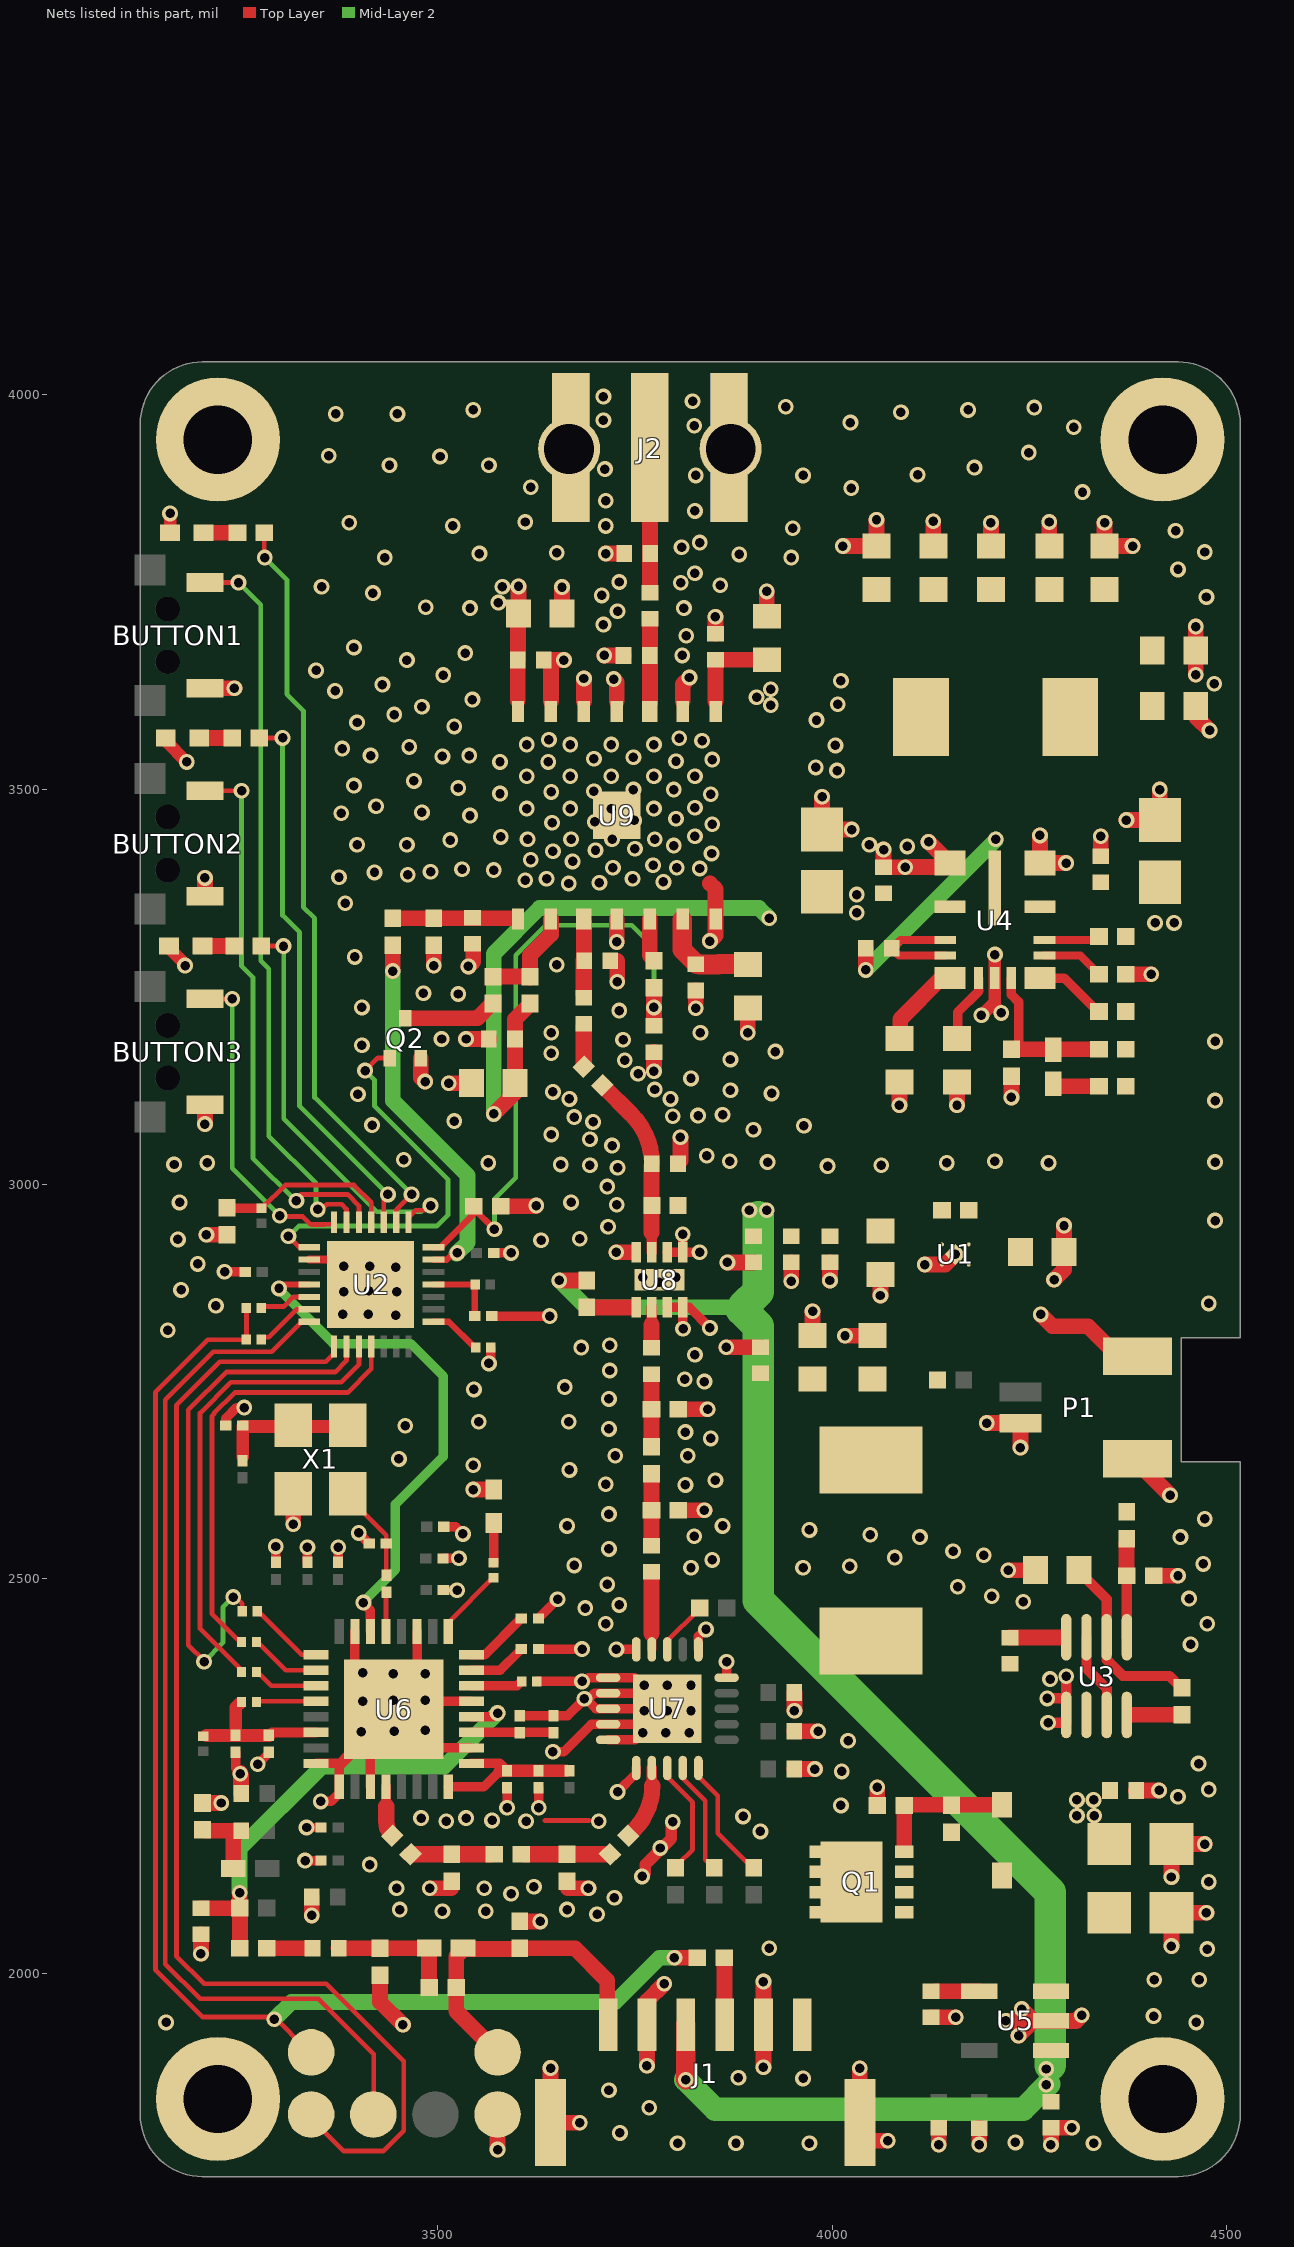
[diagram p0: the nets of this part, all layers, seen from the top]
# Altium PCB MISC62792.PcbDoc (part 2 of 2)
Units mil, origin at the board's own origin, x right, y up, seen from the top; angles counter-clockwise.
Board outline 1393.7 x 2299.21 mil, 4 copper layers (Top Layer, Mid-Layer 1, Mid-Layer 2, Bottom Layer); 176 components, 94 nets, 498 pads, 570 vias.

## Via types
v1: diameter 20, hole 12, Top Layer to Bottom Layer, tented both sides, 570 vias

## Nets (pads, with @x,y where several pads share a name; then routed paths per layer and width w, separated by ;. In a path a pad name is that pad's centre, name@x,y a point inside that pad or via, vN(x,y) a via of type N, cw(c..) or ccw(c..) an arc to the next point about the centre after c; other vN are vias at no path point) (continued)
GND: BUTTON1.1 BUTTON2.1 BUTTON3.1 C1.2 C2.2 C3.2 C4.2 C5.1 C7.1 C8.2 C9.2 C10.2 C11.2 C12.2 C13.2 C14.2 C15.2 C16.2 C17.2 C18.2 C19.2 C20.2 C21.2 C22.2 C23.2 C24.2 C25.2 C26.2 C27.2 C28.1 C29.2 C30.2 C31.1 C32.1 C33.1 C34.1 C35.2 C36.2 C37.1 C38.2 C39.1 C47.2 C50.2 C51.1 C52.2 C53.1 C54.2 C55.2 C56.1 C57.1 C58.1 C59.1 C60.1 C61.1 C62.1 C63.1 C64.2 C65.2 C67.2 C68.1 C70.1 C71.1 C72.1 C73.2 C74.2 C75.2 C76.2 C78.2 C80.1 C81.2 C82.2 C83.2 C84.2 J1.2 J1.5 J1.7 J1.8 J2.2 LED1.2 LED2.2 LED3.2 LED4.2 P1.1 P1.3 P1.4 P2.1 Q2.2 R3.1 R6.1 R12.2 R14.2 R15.2 R21.2 R25.1 R29.2 R31.2 R32.2 R33.2 R45.2 R51.2 R52.2 R53.2 SCREW1.1 SCREW2.1 SCREW3.1 SCREW4.1 SR1.2 U1.2 U1.5 U2.16 U2.29 U3.5 U4.3 U4.9 U4.11 U5.2 U6.8 U6.9 U6.11 U6.18 U6.21 U6.27 U6.31 U6.33 U7.1 U7.10 U7.11 U7.15 U7.16 U7.17 U7.18 U7.19 U7.20 U7.21 U8.3 U8.4 U8.5 U8.6 U8.8 U8.9 U9.4 U9.7 U9.9 U9.11 U9.12 U9.13 U9.15 X1.2 | length 6024.2
  Top Layer w6: 3636,2194 3692,2194
  Top Layer w10: U2.16@3337.26,2904.5 U2.29@3363.5,2904.5
  Top Layer w12: v1(3230,2889) C14.2@3256.4,2889 ; C51.1@3231.55,2694.31 3231.55,2703.31 3245.24,2717 v1(3255,2717) ; C68.1@3244,2280.2 3244,2260 v1@3250,2254 ; v1(3272,2265) 3286,2279 C67.2@3286,2280.2 ; C58.1@3295,2520.8 v1(3295,2541) ; v1(3332,2143) C53.1@3352.2,2143 ; v1(3334,2185) C52.2@3352.2,2185 ; C63.1@3335,2520.8 v1(3335,2540) ; U6.8@3346,2266.1 3376.1,2266.1 U6.33@3386,2276 ; v1(3352,2218) 3365,2218 3375.52,2228.52 U6.9@3375.52,2236.58 3375.52,2262.52 3393,2280 U6.33@3398,2280 ; C64.2@3374,2520.8 v1(3374,2540) ; U6.33@3395.21,2390.21 U6.31@3395.21,2433.42 ; v1(3400,2558.2) C47.2@3413.2,2545 ; U6.11@3414.89,2236.58 U6.33@3414.89,2274.89 ; U6.33@3473.95,2391.95 U6.27@3473.95,2433.42 ; U6.33@3503.16,2344.84 U6.21@3542.84,2344.84 ; U6.33@3504.21,2285.79 U6.18@3542.84,2285.79 ; C37.1@3506.8,2526 v1(3527,2526) ; C38.2@3507.26,2485.62 v1(3524.62,2485.62) ; C39.1@3507.8,2566 3523,2566 v1(3532,2557) ; v1(3565,2773) 3567.51,2775.51 R6.1@3567.51,2793 ; C7.1@3568.8,2833 v1(3642,2833) ; C16.2@3570.8,2913 v1(3593,2913) ; v1(3588,2210) C36.2@3588,2235.2 ; C30.2@3604,2326.8 C28.1@3647,2326.8 3664.8,2326.8 v1(3686,2348) ; R25.1@3625.51,2370 v1(3683,2370) ; C29.2@3627.8,2411 v1(3683,2411) ; C32.1@3627.8,2450 v1(3652,2474.2) ; v1(3628,2210) C34.1@3628,2235.2 ; v1(3646,2281) 3660,2281 3694.78,2315.78 U7.19@3715.9,2315.78 U7.21@3749.78,2315.78 ; v1@3687,2371 3690.83,2374.83 U7.16@3715.9,2374.83 3749.83,2374.83 U7.21@3750,2375 ; v1@3691,2345 3700.54,2335.46 U7.18@3715.9,2335.46 U7.21@3750.54,2335.46 ; v1@3693,2350 3698.15,2355.15 U7.17@3715.9,2355.15 U7.21@3750.15,2355.15 ; U7.20@3715.9,2296.09 U7.21@3750.09,2296.09 ; v1(3726.44,2410.56) U7.15@3749,2410.56 ; v1(3728,2230) 3751.63,2253.63 U7.1@3751.63,2260.36 ; U8.3@3790.84,2844.16 3818.84,2844.16 v1(3845,2818) ; U8.6@3790.84,2913.84 v1(3831.84,2913.84) ; U8.4@3810.53,2844.16 3810.53,2817.47 v1(3811,2817) ; U8.5@3810.53,2913.84 v1(3810.53,2936.53) ; U7.11@3830.37,2410.56 3830.37,2427.37 3840,2437 v1(3840,2436) ; U7.10@3866.1,2376 v1(3866.1,2394.9)
  Top Layer w13: v1(4272.41,2348.59) 4296.41,2348.59 U3.5@4296.41,2327.58 ; v1(4273.41,2317.59) 4296.41,2317.59 U3.5@4296.41,2327.58 ; v1(4296.41,2376.59) U3.5@4296.41,2327.58
  Top Layer w15: v1(3759,2123) 3763,2127 3763,2138 3796,2171 v1@3796,2189
  Top Layer w16: LED1.2@3155.61,3565.47 3155.61,3561.39 v1(3182,3535) ; LED3.2@3159.55,3301.69 3159.55,3299.45 3181,3278 v1(3180,3277) ; LED2.2@3161.05,3825.31 v1(3161.05,3849.95) ; v1(4189,3214) 4206.01,3231.01 U4.3@4206.01,3261.16 ; v1(4206.01,3290.99) U4.3@4206.01,3261.16 ; v1(4214,3217) 4206.01,3224.99 U4.3@4206.01,3261.16
  Top Layer w20: v1(3200,2025) C80.1@3200,2049.46 ; R53.2@3202,2216.04 v1(3225.96,2216.04) ; v1(3205.14,3076.14) BUTTON3.1@3205.14,3100.9 ; BUTTON2.1@3205.14,3364.68 v1(3205.14,3388.14) ; BUTTON1.1@3205.14,3628.46 v1(3242.54,3628.46) ; v1(3207.04,2935.96) SR1.2@3233,2935.96 ; v1(3250,2253) v1@3250,2254 ; C78.2@3250.88,2228 v1@3250.88,2250.88 ; v1(3317.1,2569.1) X1.2@3317.1,2608 ; v1(3340.46,2073.54) C59.1@3340.46,2097 ; R51.2@3427,1997.96 3427,1964 v1(3456,1935) ; Q2.2@3478.69,3159.61 3478.69,3135.31 v1(3484,3130) ; v1(3490.04,2107.96) R31.2@3517,2107.96 ; v1(3495,3277) R45.2@3495,3302.96 ; v1(3514,3128) C56.1@3542.9,3128 ; v1(3536,3184) C57.1@3564.92,3184 ; v1(3539,3276) 3545,3282 C5.1@3545,3303.46 ; v1(3545.19,2613.19) LED4.2@3571,2613.19 ; v1(3575.94,1776.94) P2.1@3575.94,1821.38 ; R21.2@3580.04,2972 3624,2972 v1(3625,2973) ; R52.2@3604,2066.04 v1(3629.96,2066.04) ; C54.2@3634.54,3664 v1(3660,3664) ; v1(3643.12,1880.12) J1.8@3643.12,1810.98 v1(3679.98,1810.98) ; U9.13@3643.54,3611.8 C54.2@3643.54,3658.46 ; C55.2@3657.56,3723 v1(3657.56,3756.56) ; R32.2@3665,2107.96 v1(3691.04,2107.96) ; U9.12@3685.27,3611.8 v1(3685.27,3640.73) ; v1(3711,3670) C71.1@3735.46,3670 ; v1(3713,3799) C72.1@3736.46,3799 ; v1(3723,3640) 3727,3636 U9.11@3727,3611.8 ; v1(3726.16,2913.84) U8.8@3746,2913.84 ; v1(3727,3307) U9.4@3727,3336.2 ; v1(3727.54,3256.54) C65.2@3727.54,3283 ; v1(3765.16,1883.16) J1.2@3765.16,1935 3765.16,1965.16 v1(3787,1987) ; v1(3774,3143) C70.1@3774,3167.46 ; C50.2@3807.54,3030 v1(3807.54,3059.54) ; U9.9@3810.46,3611.8 3810.46,3633.46 v1(3819,3642) ; R29.2@3813.04,2587 v1(3838,2587) ; R33.2@3814.04,2715 v1(3842,2715) ; v1(3827,3223) C74.2@3827,3245.46 ; v1(3845,3308) 3852.2,3315.2 U9.7@3852.2,3336.2 3852.2,3373.8 3845,3381 ; C76.2@3852,3697.54 v1(3852,3719) ; v1(3865.54,2793.54) C13.2@3909,2793.54 ; v1(3867.08,2900.92) C33.1@3900,2900.92 ; v1(3893,3192) C73.2@3893,3223.44 ; v1(3912.81,1881.19) J1.5@3912.81,1935 v1(3912.81,1989.81) ; C75.2@3917,3719.56 v1(3917,3751) ; v1(3948,2877) C31.1@3948,2900.92 ; C61.1@3952,2259 v1(3978,2259) ; C60.1@3952,2307 v1(3982,2307) ; v1(3952,2333) C62.1@3952,2356 ; C12.2@3975,2808.56 v1(3975,2839) ; v1(3987,3491) C15.2@3987,3449.37 v1(4024.63,3449.37) ; v1(3997,2878) C35.2@3997,2900.92 ; v1(4013.44,3808.56) C81.2@4056,3808.56 v1(4056,3842) ; v1(4016.12,2808.12) C11.2@4051,2808.12 ; v1(4034.85,1879.85) J1.7@4034.85,1810.98 4034.85,1788.15 v1(4070.15,1788.15) ; R3.1@4056.96,2213 v1(4056.96,2235.96) ; v1(4061,2859) C3.2@4061,2885.44 ; v1(4065,3424) C17.2@4065,3401.54 v1(4092.54,3401.54) ; v1(4085,3100) C2.2@4085,3129.44 ; v1@4094,3402 4144.08,3402 U4.11@4148.91,3406.84 v1(4122,3433.75) ; v1(4117.2,2898.2) U1.2@4139.07,2898.2 4143.2,2898.2 U1.5@4154,2909 ; C26.2@4125,1944.46 v1(4156.54,1944.46) ; C22.2@4128,3808.56 v1(4128,3840) ; v1(4135,1783) C25.2@4135,1804.46 ; v1(4158,3100) C84.2@4158,3129.44 ; v1(4186.33,1783.33) C24.2@4186.33,1804.18 ; v1(4195.64,2697.36) P1.1@4238.35,2697.36 v1(4238.35,2666.35) ; C82.2@4201,3808.56 v1(4201,3838) ; v1(4220,1940) U5.2@4276.93,1940 ; v1(4223,2511) C1.2@4257.44,2511 ; v1(4227,3110) R14.2@4227,3136.96 ; v1(4236,1921) U5.2@4255,1940 ; v1(4240,1955) U5.2@4255,1940 ; v1(4263.09,3441.91) U4.9@4263.09,3406.84 v1(4296.16,3406.84) ; v1(4264,2835) 4279,2820 4324,2820 4361.99,2782.01 P1.3@4386.97,2782.01 ; C20.2@4275,3808.56 v1(4275,3839) ; v1(4277,1783) C23.2@4277,1804.46 v1(4303.54,1804.46) ; v1(4281,2879) 4293.56,2891.56 C4.2@4293.56,2914 v1(4293.56,2947.56) ; v1(4316,1947) 4309,1940 U5.2@4276.93,1940 ; C18.2@4340,3415.54 v1(4340,3441) ; v1(4345,3838) C27.2@4345,3808.56 v1(4380.44,3808.56) ; R12.2@4372.04,3266 v1(4404,3266) ; v1(4372.63,3461.37) C19.2@4415,3461.37 v1(4415,3500) ; C8.2@4384.91,2232 v1(4414,2232) ; P1.4@4393.06,2646 P1.4@4386.97,2652.09 4386.97,2647.03 v1(4428,2606) ; R15.2@4407.04,2504 v1(4438,2504) ; v1(4429.74,2034.74) C10.2@4429.74,2077 v1(4474,2077) ; v1(4429.74,2122.26) C9.2@4429.74,2164 v1(4472,2164) ; C21.2@4460.56,3606 4460.56,3592.44 v1(4478,3575) ; v1(4460.56,3645.56) C83.2@4460.56,3676 v1(4460.56,3706.56) ; U5.2@4255,1940 U5.2@4276.93,1940
  other v1: 3804,1785 3878,1785 3971,1785 4331,1785 4232,1786 3731,1798 3768,1830 3717,1852 3963,1867 3881,1868 3156,1938 4461,1938 4407,1946 4408,1992 4465,1992 4475,2031 3920,2032 3702,2075 3506,2079 3561,2079 3452,2081 3664,2081 3724,2096 3593,2101 3448,2108 3559,2108 3622,2110 4477,2116 3414,2138 3782,2159 3909,2180 3798,2192 3511,2193 3612,2193 3704,2193 3569,2194 3479,2197 3536,2197 3887,2199 4011,2213 4438,2224 4477,2233 4012,2256 4464,2266 4020,2295 3760,2305 3789,2305 3819,2305 3403,2306 3445,2307 3484,2308 3762,2333 3791,2333 3821,2333 3405,2345 3444,2346 3484,2346 3762,2365 3791,2365 3821,2365 4276,2373 3444,2380 3484,2380 3405,2381 4454,2417 3713,2443 4475,2443 3687,2463 3730,2467 4242,2471 4452,2475 4202,2478 4159,2490 3715,2493 3821,2514 3963,2514 4022,2516 3673,2517 4470,2519 3848,2524 4079,2527 4192,2530 4153,2535 3717,2538 4111,2553 4441,2553 3825,2554 4048,2556 3971,2562 3664,2567 3861,2567 4472,2576 3717,2582 3814,2619 3713,2620 3852,2625 3667,2638 3545,2644 3451,2652 3725,2656 3817,2656 3846,2678 3814,2686 3717,2690 3459,2694 3552,2699 3666,2699 3717,2728 3546,2740 3661,2743 3838,2750 3813,2753 3718,2764 3826,2784 3682,2793 3718,2796 3158,2815 3447,2834 3380,2835 3412,2835 3219,2846 4477,2849 3381,2864 3448,2864 3413,2865 3175,2866 3781,2876 3760,2882 3802,2882 3447,2895 3381,2896 3414,2896 3196,2899 4156,2911 3631,2929 3171,2930 3680,2931 3716,2946 4485,2954 3727,2974 3173,2977 3669,2977 3715,2997 3728,3021 3994,3023 3693,3024 4062,3024 3166,3025 3656,3025 3208,3027 3564,3027 4145,3027 4274,3027 3918,3028 4485,3028 3870,3029 4206,3029 3457,3031 3841,3036 3721,3049 3693,3057 3644,3063 3900,3069 3964,3074 3417,3075 3697,3079 3521,3080 3673,3085 3798,3086 3830,3087 3861,3088 4485,3106 3667,3108 3795,3108 3399,3114 3923,3115 3646,3117 3871,3119 3775,3120 3821,3134 3754,3140 3737,3157 3871,3158 3644,3166 3928,3168 3404,3176 4485,3181 3735,3183 3505,3184 3644,3192 3833,3192 3730,3220 3404,3224 3526,3241 3482,3242 3651,3278 3395,3288 3383,3356 3666,3381 3705,3382 3786,3383 3611,3385 3638,3387 3747,3387 3375,3389 3462,3392 3420,3395 3491,3396 3571,3398 3531,3399 3832,3400 3722,3401 3803,3401 3773,3404 3671,3409 3618,3411 3847,3419 3646,3422 3700,3423 3750,3425 4095,3428 3799,3429 3398,3430 3461,3430 4047,3430 3516,3436 3614,3437 3669,3437 3721,3437 3775,3437 3580,3440 3826,3441 3848,3456 3645,3458 3699,3459 3749,3461 3802,3463 3541,3467 3378,3470 3480,3471 3613,3476 3668,3476 3720,3476 3774,3476 3826,3477 3422,3479 3846,3494 3579,3495 3644,3497 3698,3498 3748,3500 3799,3500 3526,3502 3394,3505 3470,3511 3613,3517 3668,3517 3720,3517 3774,3517 3826,3517 4006,3524 3979,3528 3579,3535 3640,3535 3802,3536 3848,3538 3698,3539 3748,3541 3506,3542 3415,3543 3540,3543 3379,3552 3464,3554 4004,3556 3613,3557 3668,3557 3720,3557 3774,3557 3835,3562 3641,3563 3806,3565 3521,3580 3398,3585 3980,3588 3445,3595 3480,3605 4007,3608 3544,3614 3370,3625 3430,3633 4484,3634 4011,3638 3507,3645 3346,3651 3461,3664 3810,3670 3535,3673 3394,3680 3815,3695 3710,3709 3728,3726 3541,3730 3812,3730 3485,3731 4474,3744 3708,3746 3418,3749 3353,3757 3858,3759 3808,3762 3730,3763 3826,3774 4438,3779 3433,3794 3948,3794 3882,3798 3553,3799 3651,3800 4472,3801 3809,3807 3832,3813 4435,3828 3950,3831 3519,3834 3713,3834 3388,3838 3611,3839 3826,3853 3713,3866 4317,3877 4024,3882 3618,3883 3827,3898 3963,3898 4108,3899 3712,3906 4180,3908 3439,3911 3565,3911 3503,3922 3362,3923 4249,3927 4306,3959 3825,3961 4023,3965 3710,3968 3371,3976 3449,3976 4087,3978 3545,3981 4172,3981 4256,3984 3941,3985 3823,3992 3710,3998
I_RC: P6.1 R4.2 R7.2 R8.2 | length 1715.7
  Top Layer w6: R7.2@3257.49,2803 3209,2803 3142.5,2736.5 3142.5,2404.5 3142.5,2004.5 3202,1945 3293,1945 P6.1@3335,1903 ; R7.2@3257.69,2804.69 R8.2@3257.69,2843
  Top Layer w20: v1(3800,2020) R4.2@3828.96,2020
  Mid-Layer 2 w20: v1(3293,1942) 3315,1964 3725,1964 3781,2020 v1(3800,2020)
LED1: R22.1 U2.10 | length 698.1
  Top Layer w6: R22.1@3273.84,3565.47 v1(3303.53,3565.47) ; U2.10@3431.75,2951.74 3431.75,2981.75 v1(3437,2987)
  Mid-Layer 2 w6: v1(3303.53,3565.47) 3303.53,3340.47 3325,3319 3325,3099 v1@3435,2989
LED2: R2.1 U2.9 | length 954.2
  Top Layer w6: v1@3280.47,3798.53 R2.1@3280.47,3825.31 ; U2.9@3447.5,2951.74 3447.5,2967.5 v1(3467,2987)
  Mid-Layer 2 w6: v1(3281,3794) 3309,3766 3309,3621 3330,3600 3330,3351 3344,3337 3344,3110 v1(3467,2987)
LED3: R23.1 U2.8 | length 522.2
  Top Layer w6: R23.1@3276.59,3301.69 v1(3304.69,3301.69) ; U2.8@3463.24,2951.74 3463.24,2958.24 3472,2967 3484,2967 v1@3490,2973
  Mid-Layer 2 w6: v1@3309,3299 3305,3295 3305,3083 3423,2965 3479,2965 v1@3489,2975
  other v1: 3491,2973
MUXOUT: U2.18 U6.30 | length 653.2
  Top Layer w8: v1@3304,2873 U2.18@3337.26,2873
  Top Layer w12: v1@3407,2468 3414.89,2460.11 U6.30@3414.89,2433.42
  Mid-Layer 2 w12: v1@3298.5,2867.5 3368,2798 3466,2798 3507,2757 3507,2655 3446.5,2594.5 3446.5,2511.5 v1@3407,2472 ; v1@3407,2470 v1@3408,2471
  other v1: 3406,2470 3299,2868
NetC1_1: C1.1 R5.1 U3.2 | length 230.8
  Top Layer w13: C1.1@4315,2507 4347.6,2474.4 U3.2@4347.6,2426 4347.6,2397.4 4368,2377 4427,2377 R5.1@4441,2363
NetC5_2: C5.2 R38.2 R45.1 U9.1 | length 154
  Top Layer w20: R38.2@3443,3337.04 R45.1@3495,3337.04 3572,3337.04 U9.1@3596.96,3337.04
NetC6_1: C6.1 U3.4 | length 66.5
  Top Layer w20: C6.1@4225,2425.54 U3.4@4291.46,2425.54
NetC6_2: C6.2 L2.1 U3.6
NetC7_2: C7.2 R11.1 U2.4 | length 91
  Top Layer w8: U2.4@3494.74,2872.96 R11.1@3546.96,2872.96 ; C7.2@3547.2,2833 R11.1@3547.2,2871.8
NetC26_1: C26.1 U5.4 | length 54.7
  Top Layer w20: C26.1@4131.4,1977.4 U5.4@4186.09,1977.4
NetC28_2: C28.2 C30.1 U6.19 | length 103.7
  Top Layer w12: U6.19@3542.84,2305.47 C28.2@3646.53,2305.47
NetC29_1: C29.1 U6.23 | length 71.4
  Top Layer w12: U6.23@3542.84,2384.21 3579.21,2384.21 C29.1@3604,2409
NetC32_2: C32.2 U6.24 | length 80.8
  Top Layer w12: U6.24@3542.84,2403.9 3559.9,2403.9 C32.2@3605,2449
NetC34_2: C34.2 C36.1 L26.2 U6.16 U6.17 | length 204
  Top Layer w12: U6.16@3513.32,2236.58 3558.58,2236.58 3578.73,2256.73 ; U6.17@3542.84,2266.1 3578.9,2266.1 C36.1@3586,2259
  Top Layer w16: 3579,2256.45 3579.35,2256.8 C36.1@3588,2256.8 C34.2@3628,2256.8 L26.2@3663,2256.8
NetC41_1: C41.1 U6.29 | length 48
  Top Layer w6: U6.29@3434.58,2433.42 C41.1@3434.58,2481.42
NetC41_2: C41.2 C47.1 X1.3 | length 96.8
  Top Layer w6: X1.3@3402,2588 3434.8,2555.2 C47.1@3434.8,2545 ; C41.2@3435,2504.8 C47.1@3435,2545
NetC42_1: C42.1 U6.12 | length 96.5
  Top Layer w13: 3434.58,2217.58 U6.12@3434.58,2236.58
  Top Layer w20.56: 3435,2211.5 3435,2192.33 ccw(c3459.94,2192.33) C42.1@3442.3,2174.7 ; C42.1@3442.3,2174.7 cw(c3459.74,2192.13) 3435.08,2192.13 ccw(c3459.74,2192.13) C42.1@3442.3,2174.7
NetC42_2: C42.2 R30.1 R31.1 | length 101
  Top Layer w20.56: C42.2@3466,2151 R30.1@3567,2151
NetC43_1: C43.1 R30.2 R32.1 | length 105.9
  Top Layer w20.56: R30.2@3610.09,2151 C43.1@3716,2151
NetC43_2: C43.2 U7.2 | length 81.6
  Top Layer w13: 3771.32,2241.36 U7.2@3771.32,2260.36
  Top Layer w20.56: 3748.67,2181.67 ccw(c3692.33,2238) 3772,2238
NetC44_1: C44.1 U7.14 | length 90
  Top Layer w12: U7.14@3771.32,2410.56 3771.32,2429.56
  Top Layer w20.56: 3771,2431 C44.1@3771,2502
NetC44_2: C44.2 R27.1 R29.1 | length 84
  Top Layer w20.56: C44.2@3771,2547 R27.1@3771,2631
NetC45_1: C45.1 R27.2 R33.1 | length 84
  Top Layer w20.56: R27.2@3771,2672 C45.1@3771,2756
NetC45_2: C45.2 U8.2 | length 44
  Top Layer w13: 3771.16,2825.16 U8.2@3771.16,2844.16
  Top Layer w20.56: C45.2@3771,2797 3771,2822
NetC46_1: C46.1 C50.1 L4.1 U8.7 | length 289.9
  Top Layer w13: U8.7@3771.16,2913.84 3771.16,2930.84
  Top Layer w20.56: C46.1@3710,3124 3745.62,3088.38 ; 3771,2939 C50.1@3771,3023 ; 3745.62,3088.38 cw(c3683.24,3026) C50.1@3771.46,3026 ccw(c3683.24,3026) 3745.62,3088.38
NetC46_2: C46.2 C66.2 | length 49.8
  Top Layer w20.56: C46.2@3685,3150.24 3685,3181 C66.2@3685,3200
NetC51_2: C51.2 R39.2 X1.1 X1.4 | length 157
  Top Layer w16: R39.2@3253,2655 3253,2693 X1.4@3372,2693
NetC65_1: C65.1 C66.1 U9.3 | length 90
  Top Layer w20.56: C66.1@3685,3241 U9.3@3685.27,3331
NetC67_1: C67.1 C68.2 R43.2 R47.1 U6.6 | length 182.2
  Top Layer w13: C67.1@3287,2302 3290.47,2305.47 U6.6@3346,2305.47
  Top Layer w16: R47.1@3207,2301.51 C67.1@3286.51,2301.51 ; C68.2@3244,2301.8 3244,2337 R43.2@3249,2342
NetC69_1: C69.1 C71.2 U9.10 | length 104
  Top Layer w20.56: U9.10@3769,3610 C69.1@3769,3714
NetC69_2: C69.2 C72.2 J2.1 | length 175.6
  Top Layer w20.56: C69.2@3769,3757 J2.1@3769,3932.58
NetC77_1: C77.1 C87.2 R50.1 R51.1 | length 157.7
  Top Layer w20: C77.1@3374.54,2032 C87.2@3488,2032 ; R50.1@3489.17,1988.17 C87.2@3489.17,2032.41
NetC77_2: C77.2 R19.2 | length 52.5
  Top Layer w20: R19.2@3283.46,2032 C77.2@3336,2032
NetC79_1: C79.1 C88.1 R53.1 | length 93.3
  Top Layer w20: R53.1@3207,2181 3249,2181 3240.96,2172.96 C88.1@3240.96,2133
NetC84_1: C84.1 U4.2 | length 79.1
  Top Layer w12: C84.1@4159,3193 4159,3218 4185.34,3244.34 U4.2@4185.34,3261.16
NetC85_1: C85.1 U4.13 U4.14 | length 134.7
  Top Layer w10: C85.1@4078,3301 4086.39,3309.39 U4.13@4143.01,3309.39 ; C85.1@4079,3295 4084.29,3289.71 U4.14@4143.01,3289.71
NetC85_2: C85.2 L3.1 U4.10 | length 261.2
  Top Layer w20: v1(4042.46,3271.46) C85.2@4042.46,3299
  Mid-Layer 2 w20: v1(4042.46,3271.46) 4207,3436 v1(4207,3437)
NetC86_1: C86.1 R14.1 R16.2 U4.4 | length 207
  Top Layer w12: U4.4@4226.68,3261.16 4226.68,3240.32 4236,3231 4236,3179 4231,3174 R14.1@4228,3174 ; R14.1@4227,3171.04 R14.1@4228.78,3173.41
  Top Layer w20: R14.1@4227,3171.04 R16.2@4334.96,3171.04
NetC86_2: C86.2 R17.2 | length 55
  Top Layer w20: C86.2@4283,3124 R17.2@4337.96,3124
NetJ1_4: J1.4 R4.1 | length 78.4
  Top Layer w20: J1.4@3863.59,1935 R4.1@3863.59,2013.41
NetJ1_6: J1.6 Q1.5 Q1.6 Q1.7 Q1.8 Q1.9
NetLED1_1: LED1.1 R22.2 | length 34.5
  Top Layer w20: LED1.1@3197.99,3565.47 R22.2@3232.53,3565.47
NetLED2_1: LED2.1 R2.2 | length 38.9
  Top Layer w20: LED2.1@3203.43,3825.31 R2.2@3242.31,3825.31
NetLED3_1: LED3.1 R23.2 | length 35.4
  Top Layer w20: LED3.1@3201.93,3301.69 R23.2@3237.31,3301.69
NetLED4_1: LED4.1 R28.1 | length 42.5
  Top Layer w12: R28.1@3571,2520.51 LED4.1@3571,2563
NetQ1_4: Q1.4 R1.1 R3.2 ZD1.1 | length 176.1
  Top Layer w20: Q1.4@4091.04,2159.04 R3.2@4091.04,2213 ; R3.2@4092.88,2213.88 ZD1.1@4215,2213.88
NetQ2_3: Q2.3 R26.2 | length 111
  Top Layer w20: Q2.3@3463,3210.4 3548.22,3210.4 3548.22,3210.63 3550.63,3210.63 R26.2@3567,3227
NetR5_2: R5.2 U3.8 | length 62
  Top Layer w20: 4381.04,2327.96 R5.2@4443,2327.96
NetR6_2: R6.2 U2.1 | length 64.4
  Top Layer w8: U2.1@3494.74,2825.76 3514.24,2825.76 R6.2@3546,2794
NetR7_1: R7.1 U2.20 | length 74
  Top Layer w6: R7.1@3278,2806 3286,2806 3321.5,2841.5 U2.20@3337.26,2841.5
NetR8_1: R8.1 U2.19 | length 62.3
  Top Layer w6: R8.1@3280,2845 3305,2845 3317.26,2857.26 U2.19@3337.26,2857.26
NetR9_1: R9.1 U4.5 | length 89
  Top Layer w12: U4.5@4263.09,3261.16 4267.84,3261.16 4293.84,3261.16 R9.1@4335,3220
NetR10_2: R10.2 R15.1 U3.1 | length 112.4
  Top Layer w13: U3.1@4373.19,2426 R15.1@4373.19,2502.19
  Top Layer w20: R15.1@4372.8,2508.79 R10.2@4372.8,2545
NetR12_1: R12.1 U4.6 | length 77.4
  Top Layer w10: U4.6@4268.99,3289.71 4314.29,3289.71 R12.1@4337,3267
NetR13_1: R13.1 U4.7 | length 65.4
  Top Layer w10: U4.7@4268.99,3309.39 R13.1@4334.39,3309.39
NetR18_2: R18.2 SR1.1 U2.11 | length 233.4
  Top Layer w6: SR1.1@3230,2972 3232.49,2969.51 SR1.1@3234.49,2969.51 ; R18.2@3277,2970 3278,2970 3307,2999 3394,2999 3416,2977 U2.11@3416,2951.71
  Top Layer w12: SR1.1@3234.49,2969.51 R18.2@3277,2969.51
NetR24_2: R24.2 U8.1 | length 58
  Top Layer w20: R24.2@3689,2843.96 U8.1@3746.96,2843.96
NetR25_2: R25.2 U6.22 | length 64
  Top Layer w12: U6.22@3542.84,2364.53 3600.53,2364.53 R25.2@3605,2369
NetR26_1: R26.1 R46.2 U9.2 | length 129.2
  Top Layer w20: R26.1@3570,3263.04 R46.2@3613.96,3263.04 ; R46.2@3617,3262 R46.2@3617,3263.04 3617,3290 3643.54,3316.54 U9.2@3643.54,3336.2
NetR28_2: R28.2 U6.25 | length 93.9
  Top Layer w6: U6.25@3513.32,2433.42 3513.32,2444.32 R28.2@3572,2503
NetR34_1: R34.1 U7.3 | length 142.1
  Top Layer w6: U7.3@3791,2260.36 3791,2249 3823,2217 3823,2157 R34.1@3805,2139
NetR35_1: R35.1 U7.13 | length 66
  Top Layer w6: U7.13@3791,2410.56 3791,2421.43 R35.1@3830,2460.43
NetR36_1: R36.1 U7.4 | length 139.4
  Top Layer w6: U7.4@3810.69,2260.36 3810.69,2247.31 3839,2219 3839,2144 R36.1@3847,2136
NetR37_1: R37.1 U7.5 | length 152
  Top Layer w6: U7.5@3830.37,2260.36 3830.37,2249.63 3855,2225 3855,2178 R37.1@3897,2136
NetR40_1: R40.1 U6.1 | length 95.8
  Top Layer w6: R40.1@3273,2459 3328.1,2403.9 U6.1@3346,2403.9
NetR41_1: R41.1 U6.2 | length 88.8
  Top Layer w6: R41.1@3272,2420 3307.78,2384.22 U6.2@3346,2384.22
NetR42_1: R42.1 U6.3 | length 79.8
  Top Layer w6: R42.1@3273,2381 3289.47,2364.53 U6.3@3346,2364.53
NetR43_1: R43.1 U6.4 | length 71.8
  Top Layer w6: R43.1@3274.16,2344.84 U6.4@3346,2344.84
NetR48_2: R48.2 U9.5 | length 53.4
  Top Layer w20: U9.5@3768.73,3336.2 3768.73,3307 3768.73,3290.27 R48.2@3774,3285
ON/OFF: Q2.1 U2.15 | length 507.3
  Top Layer w6: v1(3311,2934) 3324.76,2920.24 U2.15@3337.26,2920.24 ; v1(3408,3144) 3424,3160 Q2.1@3437,3160
  Mid-Layer 2 w6: v1(3311,2934) 3324,2947 3499,2947 3513,2961 3513,3006 3420,3099 3420,3132 v1(3408,3144)
PA_5.5V: C2.1 C20.1 C21.1 C22.1 C27.1 C54.1 C55.1 C56.2 C57.2 C73.1 C74.1 C75.1 C76.1 C81.1 C82.1 C83.1 L3.2 R9.2 R16.1 R17.1 R46.1 U4.1 U9.6 U9.8 U9.14 | length 1227.4
  Top Layer w20: v1(3571,3089) 3598.02,3116.02 C56.2@3598.02,3128 ; C56.2@3598,3132 3598,3209 R46.1@3617,3228 ; 3601.46,3612.54 C54.1@3601.46,3664 ; C54.1@3601.8,3664 C55.1@3601.8,3715.2 ; C55.1@3602.44,3723 v1(3602.44,3757.44) ; C76.1@3852,3664.46 C75.1@3916.46,3664.46 ; U9.8@3852.2,3611.8 C76.1@3852.2,3662.8 ; C2.1@4086,3184 4086,3209 4138.16,3261.16 U4.1@4148.91,3261.16
  Top Layer w25: U9.6@3810,3335 3810,3297 3828,3279 3831.7,3279 3832.2,3278.5 3855.8,3278.5 3856.3,3279 C73.1@3894,3279
  Mid-Layer 2 w20: v1(3571,3089) 3571,3292 3629,3350 3907,3350 v1(3920,3337)
  other v1: 3922,3607 3904,3617 3922,3627 3577,3737 3582,3757
POWER-IN: C8.1 C9.1 C10.1 C15.1 C17.1 C18.1 C19.1 Q1.1 Q1.2 Q1.3 R1.2 R13.2 U3.3 U3.7 U4.8 U4.12 ZD1.2 | length 91.8
  Top Layer w13: U3.3@4322,2426 4322,2387 4348,2361 U3.7@4348,2345
  other v1: 4310,2200 4332,2200 4310,2220 4331,2220 4409,3331 4433,3331 4031,3344 4031,3367
"SPI LE": R42.2 U2.24 | length 593.3
  Top Layer w6: R42.2@3249,2387 3199,2437 3199,2710 3238,2749 3378,2749 3400.26,2771.26 U2.24@3400.26,2794.26
SPICLK: R40.2 U2.23 | length 690.4
  Top Layer w6: 3184,2485 3184,2488 ; v1(3204,2395) 3204,2396 3184,2416 3184,2488 ; v1@3246,2475 3252.49,2468.51 R40.2@3252.49,2459 ; U2.23@3384.5,2794.26 3384.5,2776.5 3370,2762 3232,2762 3184,2714 3184,2488
  Mid-Layer 2 w6: v1(3204,2395) 3228,2419 3228,2464 v1(3241,2477)
SPIDATA: R41.2 U2.25 | length 552.4
  Top Layer w6: R41.2@3247,2423 3214,2456 3214,2706 3216.55,2708.55 3216.55,2709.52 3243.03,2736 3386,2736 3416,2766 U2.25@3416,2794.27
SW1_BAND: BUTTON1.2 U2.13 | length 946.2
  Top Layer w6: BUTTON1.2@3205.14,3762.32 v1(3247.68,3762.32) ; v1(3348,2968) 3353,2968 3359.52,2974.52 3378.48,2974.52 3384.5,2968.5 U2.13@3384.5,2951.74
  Mid-Layer 2 w6: v1@3249,3761 3276,3734 3276,3283 3286,3273 3286,3061 3346,3001 3346,2967 3352,2967 3352,2968 v1(3348,2968)
SW1_FRE: BUTTON2.2 U2.12 | length 706.8
  Top Layer w6: BUTTON2.2@3205.14,3498.54 v1(3251.54,3498.54) ; v1@3319,2979 3327,2987 3386,2987 3400.26,2972.74 U2.12@3400.26,2951.74 ; v1(3321,2979) v1@3321,2980
  Mid-Layer 2 w6: v1(3251.54,3498.54) 3251.54,3276.46 3266,3262 3266,3244 3266,3240 3266,3033 v1@3320,2979
SW1_POWER: BUTTON3.2 U2.14 | length 407.7
  Top Layer w6: BUTTON3.2@3205.14,3234.76 v1(3239.76,3234.76) ; v1@3303,2961 3305,2959 3329,2959 3338.76,2949.24 3339.89,2949.24 3340.13,2949 3355.87,2949 3356.11,2949.24 3368.76,2949.24 U2.14@3368.76,2951.74
  Mid-Layer 2 w6: v1(3239.76,3234.76) 3239.76,3020.24 3262,2998 v1(3300,2960)
SWCLK: P5.1 U2.22 | length 1489.5
  Top Layer w6: P5.1@3354,1802 3381,1775 3431,1775 3456.99,1800.99 3456.99,1849.01 3457,1889 3359,1987 3204,1987 3169,2022 3169,2720 3224,2775 3358,2775 3368.76,2785.76 U2.22@3368.76,2794.26
SWDIO: P4.1 U2.21 | length 1322.6
  Top Layer w6: U2.21@3337.26,2825.76 3327.76,2825.76 3289.62,2787.62 3215.62,2787.62 3155,2727 3155,2012 3199,1968 3349,1968 3419,1898 3419,1829 P4.1@3416,1826
VCC_5V: C3.1 C23.1 C31.2 C33.2 C35.1 J1.3 L4.2 R20.1 R24.1 U1.1 U5.1 U5.3 | length 2086.7
  Top Layer w20: v1(3654.04,2878.04) R24.1@3689,2878.04
  Top Layer w25: v1(3814.37,1865.37) J1.3@3814.37,1935
  Mid-Layer 2 w20: v1(3654.04,2878.04) 3688.08,2844 3888,2844
  Mid-Layer 2 w30: v1(3814.37,1865.37) 3851.73,1828 4242,1828 v1@4274,1860
  Mid-Layer 2 w40: 3906,2959 3906,2864 3888,2846 3888,2844 3885,2841 3906,2820 3906,2473 4276,2103 v1@4276,1884
  other v1: 4271,1859 4271,1879 3895,2967 3917,2967
VCC_5V3: C4.1 C11.1 C12.1 C13.1 L1.2 L2.2 R10.1 R20.2 U1.3 U1.4
VDET: C70.2 R21.1 R48.1 U2.7 | length 795.7
  Top Layer w8: U2.7@3494.74,2920.24 3504.24,2920.24 3504.95,2920.95 3504.95,2921.28 3548,2964.34 R21.1@3548,2973 ; R21.1@3545.96,2972 3545.96,2969.04 v1(3572,2943)
  Top Layer w20: C70.2@3774,3205 v1(3774,3224) R48.1@3774,3248.96
  Mid-Layer 2 w6: v1@3572,2948 3572,2981 3599,3008 3599,3290 3637,3328 3746,3328 3774,3300 v1(3774,3224)
VIDEO-IN: C87.1 J1.1 P7.1 R50.2 R52.1 | length 402
  Top Layer w20: P7.1@3570,1906 3523.67,1952.33 R50.2@3523.67,1982.41 3523.67,2021.67 3533,2031 R52.1@3600,2031 ; R52.1@3604,2031.96 3674.04,2031.96 3715,1991 J1.1@3715,1932
VREF: R38.1 U2.6 | length 481.2
  Top Layer w8: U2.6@3494.74,2904.5 3511.5,2904.5 3524,2917 3524.52,2917 3524.95,2916.57 v1(3524.95,2913) ; v1(3524.95,2913) 3524.95,2912.72 3525,2912.72 3525,2913 v1(3524.95,2913)
  Top Layer w20: v1(3443,3270) R38.1@3443,3302.96
  Mid-Layer 2 w8: v1@3524.52,2917.48 3524.52,2917 3524.95,2916.57 v1(3524.95,2913) ; v1(3524.95,2913) 3524.95,2912.95 3524.95,2912.72 3525,2912.72 3525,2913 v1(3524.95,2913)
  Mid-Layer 2 w20: v1(3443,3270) 3443,3106 3538,3011 3538,2926 3525,2913 3524.95,2912.95 v1@3524,2912
VTUNE: C80.2 R19.1 R49.2 U6.20 | length 602.9
  Top Layer w12: U6.20@3542.84,2325.16 3571.16,2325.16 v1(3576,2330)
  Top Layer w20: C80.2@3200,2082.54 3249.54,2082.54 3249.54,2057 ; R49.2@3249.38,2083 v1(3249.38,2102.38) ; R19.1@3249.54,2037.46 3249.54,2057 ; 3250,2057 3249.54,2057
  Mid-Layer 2 w20: v1@3249,2103 3249,2158 3353,2262 3508,2262 v1(3576,2330)
pads on no net: BUTTON1.0 BUTTON1.3 BUTTON1.4 BUTTON2.0 BUTTON2.3 BUTTON2.4 BUTTON3.0 BUTTON3.3 BUTTON3.4 U2.2 U2.3 U6.5 U6.13 U6.14 U6.15 U6.26 U7.6 U7.7 U7.8 U7.12

## Polygon pours and split planes (outlines as drawn)
PA_5.5V on Top Layer "Bottom Layer-No Net" (solid, remove dead copper, pour order 1001): 3566,3755 3566,3598 3574,3590 3579,3585 3594,3585 3609,3585 3611,3587 3612,3588 3612,3629 3612,3696 3620,3704 3620,3721 3620,3770 3612,3778 3608,3782 3602,3782 3580,3782 3575,3777 3566,3768 3566,3755
PA_5.5V on Top Layer "Bottom Layer-No Net" (solid, remove dead copper, pour order 1000): 3840,3668 3840,3648 3840,3591 3843,3588 3844,3587 3854,3587 3933,3587 3936,3590 3942,3596 3942,3604 3942,3606 3962,3626 4024,3688 4081,3688 4223,3688 4230,3695 4230,3696 4230,3751 4222,3759 4206,3775 4154,3775 3985,3775 3962,3752 3956,3746 3956,3716 3956,3708 3944,3696 3933,3685 3910,3685 3880,3685 3874,3679 3871,3676 3859,3676 3843,3676 3841,3674 3840,3673 3840,3669
GND on Top Layer "Bottom Layer-No Net" (solid, remove dead copper, pour order 1011): 3050.39,3815 3056.39,3809 3056.39,1835 3056.39,1716 3116.39,1656 3165.39,1607 3327.39,1607 4613.39,1607 4678.39,1672 4705.39,1699 4705.39,1743 4705.39,3945 4651.39,3999 4531.39,4119 4260.39,4119 3181.39,4119 3067.39,4005 3045.39,3983 3045.39,3826
PA_5.5V on Top Layer "Bottom Layer-No Net" (solid, remove dead copper, pour order 1010): 3871,3293 3871,3266 3876,3261 3877,3260 3886,3260 3938,3260 4027,3171 4031,3167 4075,3167 4099,3167 4104,3172 4108,3176 4108,3180 4108,3203 4103,3208 4099,3212 4093,3212 4046,3212 4028,3230 3942,3316 3942,3372 3942,3493 3942,3612 3961,3631 4018,3688 4199,3688 4225,3688 4255,3658 4259,3654 4259,3635 4259,3544 4272,3531 4277,3526 4290,3526 4434,3526 4458,3502 4465,3495 4465,3480 4465,3252 4448,3235 4446,3233 4433,3233 4366,3233 4363,3230 4362,3229 4362,3224 4362,3113 4364,3111 4366,3109 4369,3109 4399,3109 4402,3112 4404,3114 4404,3120 4404,3187 4412,3195 4420,3203 4432,3203 4453,3203 4465,3215 4492,3242 4492,3511 4492,3518 4435,3575 4421,3589 4421,3705 4421,3741 4393,3769 4388,3774 4369,3774 4022,3774 3946,3698 3933,3685 3917,3685 3905,3685 3900,3680 3883,3663 3883,3364 3883,3323 3873,3313 3871,3311 3871,3294
NetC85_2 on Top Layer "Bottom Layer-No Net" (solid, remove dead copper, pour order 1009): 4041,3616 4041,3490 4055,3476 4068,3463 4105,3463 4163,3463 4174,3452 4182,3444 4182,3395 4182,3330 4186,3326 4189,3323 4204,3323 4224,3323 4227,3326 4230,3329 4230,3358 4230,3498 4207,3521 4175,3553 4175,3603 4175,3635 4163,3647 4158,3652 4139,3652 4056,3652 4043,3639 4041,3637 4041,3616
POWER-IN on Top Layer "Bottom Layer-No Net" (solid, remove dead copper, pour order 1008): 4242,3356 4242,3342 4244,3340 4249,3335 4275,3335 4352,3335 4356,3331 4361,3326 4361,3314 4361,3303 4363,3301 4365,3299 4438,3299 4449,3310 4455,3316 4455,3345 4455,3397 4445,3407 4441,3411 4433,3411 4383,3411 4373,3401 4365,3393 4339,3393 4326,3393 4314,3381 4299,3366 4266,3366 4246,3366 4244,3364 4242,3362 4242,3357
POWER-IN on Top Layer "Bottom Layer-No Net" (solid, remove dead copper, pour order 1007): 3956,3381 3956,3345 3959,3342 3973,3328 4124,3328 4164,3328 4168,3332 4170,3334 4170,3345 4170,3359 4167,3362 4165,3364 4151,3364 4106,3364 4095,3375 4090,3380 4062,3380 4042,3380 4024,3398 4021,3401 3996,3401 3963,3401 3958,3396 3956,3394 3956,3381
3.3V on Top Layer "Bottom Layer-No Net" (solid, remove dead copper, pour order 1006): 4120,1869 4120,1832 4124,1828 4125,1827 4128,1827 4204,1827 4206,1829 4210,1833 4210,1892 4210,1911 4208,1913 4206,1915 4201,1915 4135,1915 4127,1907 4120,1900 4120,1870
VCC_5V on Top Layer "Bottom Layer-No Net" (solid, remove dead copper, pour order 1005): 4250,1897 4250,1837 4255,1832 4259,1828 4272,1828 4306,1828 4310,1832 4321,1843 4321,1857 4321,1886 4341,1906 4356,1921 4356,1937 4356,1975 4342,1989 4336,1995 4328,1995 4257,1995 4255,1993 4253,1991 4253,1985 4253,1969 4255,1967 4256,1966 4267,1966 4307,1966 4311,1970 4312,1971 4317,1971 4329,1971 4334,1966 4341,1959 4341,1949 4341,1934 4326,1919 4320,1913 4287,1913 4255,1913 4253,1911 4250,1908 4250,1898
VCC_5V3 on Top Layer "Bottom Layer-No Net" (solid, remove dead copper, pour order 1004): 4162,2966 4162,2931 4171,2922 4175,2918 4175,2909 4175,2903 4175,2902 4095,2822 4088,2815 4088,2801 4088,2785 4080,2777 4073,2770 3986,2770 3899,2770 3890,2761 3886,2757 3886,2731 3886,2647 3915,2618 3933,2600 4107,2600 4140,2600 4158,2582 4167,2573 4373,2573 4385,2573 4388,2576 4391,2579 4391,2583 4391,2600 4387,2604 4386,2605 4372,2605 4211,2605 4180,2636 4145,2671 4145,2755 4145,2801 4160,2816 4207,2863 4230,2863 4248,2881 4255,2888 4255,2913 4255,2950 4238,2967 4221,2984 4197,2984 4168,2984 4164,2980 4162,2978 4162,2966
VCC_5V on Top Layer "Bottom Layer-No Net" (solid, remove dead copper, pour order 1003): 3804,2975 3804,2956 3805,2955 3807,2953 3817,2953 3867,2953 3873,2947 3878,2942 3878,2935 3878,2930 3882,2926 3884,2924 3895,2924 4086,2924 4091,2919 4132,2919 4139,2919 4142,2922 4150,2930 4150,2956 4150,2980 4146,2984 4142,2988 4129,2988 3808,2988 3807,2987 3804,2984 3804,2975
+5V-FAN on Top Layer "Bottom Layer-No Net" (solid, remove dead copper, pour order 1002): 4155,2757 4155,2733 4159,2729 4164,2724 4214,2724 4263,2724 4267,2728 4270,2731 4270,2733 4270,2767 4266,2771 4262,2775 4248,2775 4165,2775 4156,2766 4155,2765 4155,2758
NetC6_2 on Top Layer "Bottom Layer-No Net" (solid, remove dead copper, pour order 1001): 3975,2442 3975,2366 3981,2360 3987,2354 4019,2354 4051,2354 4067,2338 4076,2329 4076,2305 4076,2283 4109,2250 4117,2242 4206,2242 4297,2242 4316,2261 4332,2277 4332,2329 4332,2356 4328,2360 4324,2360 4317,2360 4314,2357 4312,2355 4312,2346 4312,2296 4304,2288 4301,2285 4293,2285 4261,2285 4251,2295 4248,2298 4248,2371 4248,2397 4244,2401 4243,2402 4235,2402 4198,2402 4174,2426 4124,2476 4094,2476 3992,2476 3983,2467 3975,2459 3975,2443
POWER-IN on Top Layer "Bottom Layer-No Net" (solid, remove dead copper, pour order 1000): 4078,2128 4078,2049 4084,2043 4097,2030 4144,2030 4361,2030 4371,2040 4379,2048 4379,2076 4379,2205 4365,2219 4363,2221 4363,2248 4363,2286 4358,2291 4357,2292 4357,2301 4357,2355 4355,2357 4354,2358 4353,2358 4343,2358 4341,2356 4340,2355 4340,2348 4340,2265 4330,2255 4297,2222 4297,2185 4297,2176 4281,2160 4267,2146 4240,2146 4189,2146 4184,2151 4174,2161 4174,2176 4174,2183 4169,2188 4167,2190 4158,2190 4140,2190 4137,2187 4133,2183 4133,2175 4133,2153 4126,2146 4117,2137 4095,2137 4080,2137 4079,2136 4078,2135 4078,2129
NetJ1_6 on Top Layer "Bottom Layer-No Net" (solid, remove dead copper, pour order 1000): 3949,1966 3949,1945 3949,1901 3950,1900 3951,1899 3953,1899 4001,1899 4005,1903 4007,1905 4007,1920 4007,1969 4049,2011 4064,2026 4064,2074 4064,2167 4061,2170 4060,2171 4050,2171 3972,2171 3966,2165 3964,2163 3964,2148 3964,2021 3961,2018 3949,2006 3949,1966
PA_5.5V on Mid-Layer 2 "Bottom Layer-No Net" (solid, remove dead copper, pour order 1000): 3567,3767 3567,3757 3567,3627 3606,3588 3614,3580 3627,3580 3926,3580 3935,3589 3937,3591 3937,3596 3937,3637 3932,3642 3931,3643 3928,3643 3907,3643 3901,3637 3887,3623 3818,3623 3660,3623 3629,3654 3620,3663 3620,3693 3620,3767 3612,3775 3610,3777 3603,3777 3576,3777 3569,3770 3567,3768 3567,3767
GND on Mid-Layer 2 "Bottom Layer-No Net" (solid, remove dead copper, pour order 1016): 2983.28,3732.34 2983.28,1797.34 3081.28,1699.34 3106.28,1674.34 3333.28,1674.34 4572.28,1674.34 4656.28,1758.34 4710.28,1812.34 4710.28,2029.34 4710.28,3949.34 4552.28,4107.34 4508.28,4151.34 4389.28,4151.34 3136.28,4151.34 3067.28,4082.34 2978.28,3993.34 2978.28,3756.34
POWER-IN on Mid-Layer 2 "Bottom Layer-No Net" (solid, remove dead copper, pour order 1015): 3959,3362 3959,3131 4001,3089 4026,3064 4103,3064 4296,3064 4312,3048 4320,3040 4320,3003 4320,2881 4298,2859 4288,2849 4288,2836 4288,2464 4315,2437 4322,2430 4322,2357 4322,2305 4298,2281 4287,2270 4287,2221 4287,2200 4295,2192 4301,2186 4315,2186 4369,2186 4379,2196 4385,2202 4385,2207 4385,2241 4412,2268 4425,2281 4425,2305 4425,2458 4410,2473 4394,2489 4394,2788 4394,2815 4424,2845 4461,2882 4461,3302 4461,3336 4453,3344 4448,3349 4441,3349 4322,3349 4301,3328 4301,3242 4301,3225 4272,3196 4262,3186 4229,3186 4079,3186 4058,3207 4018,3247 4018,3274 4018,3295 4040,3317 4050,3327 4050,3337 4050,3374 4043,3381 4038,3386 4031,3386 3982,3386 3959,3363
VCC_5V on Mid-Layer 2 "Bottom Layer-No Net" (solid, remove dead copper, pour order 1014): 4255,1884 4255,1863 4255,1854 4259,1850 4264,1845 4269,1845 4289,1845 4291,1847 4296,1852 4296,1882 4296,1895 4293,1898 4291,1900 4282,1900 4260,1900 4258,1898 4255,1895 4255,1885
VCC_5V on Mid-Layer 2 "Bottom Layer-No Net" (solid, remove dead copper, pour order 1013): 3883,2975 3883,2957 3887,2953 3889,2951 3895,2951 3925,2951 3928,2954 3930,2956 3930,2961 3930,2977 3926,2981 3925,2982 3913,2982 3890,2982 3883,2975
3.3V on Mid-Layer 2 "Bottom Layer-No Net" (solid, remove dead copper, pour order 1012): 4114,1903 4114,1870 4119,1865 4125,1859 4135,1859 4152,1859 4158,1865 4165,1872 4165,1879 4165,1904 4156,1913 4151,1918 4149,1918 4125,1918 4122,1915 4114,1907 4114,1904
GND on Bottom Layer "Bottom Layer-No Net" (solid, remove dead copper, pour order 1017): 2946,3765 2946,1841 3104,1683 3144,1643 3449,1643 4634,1643 4703,1712 4757,1766 4757,2018 4757,3934 4565,4126 4526,4165 4195,4165 3114,4165 3020,4071 2946,3997 2946,3790
GND on Mid-Layer 1 "Bottom Layer-No Net" (solid, remove dead copper, pour order 1018): 3038,3841 3038,1740 3109,1669 3329,1669 4550,1669 4597,1716 4746,1865 4746,2086 4746,3927 4541,4132 4439,4234 4046,4234 3202,4234 3077,4109 3034,4066 3034,3841

## Keep-outs
Keep-Out Layer:
  the board outline again, w3.94

## Other copper
Mid-Layer 1:
  pour cut-out: 3725,3838 3813,3838 3813,4037 3726,4037 3725,4038

## Silkscreen, mask and mechanical layers (free items; w line width, h text height)
Top Overlay:
  lines w3.94: 3123.45,3006.68 3709.8,3006.68 3709.8,3046.7 3124.1,3046.7 ; 4516.63,3006.68 3847.6,3006.68 3847.6,3046.7 4516.89,3046.7
  text "CLK" at 3301,1756 h40
  text "3.3V" at 3463,1756 h40
  text "DIO" at 3391,1755 h40
  text "GND" at 3542,1755 h40
Top Solder:
  rectangle: 3123.19,3006.42 3711.2,3045.79
  rectangle: 3847.6,3002.48 4516.89,3049.72
Bottom Solder:
  region: 129 vertices and 40 holes, not listed, extent 3145.34,1764.79 4494.74,4019.7